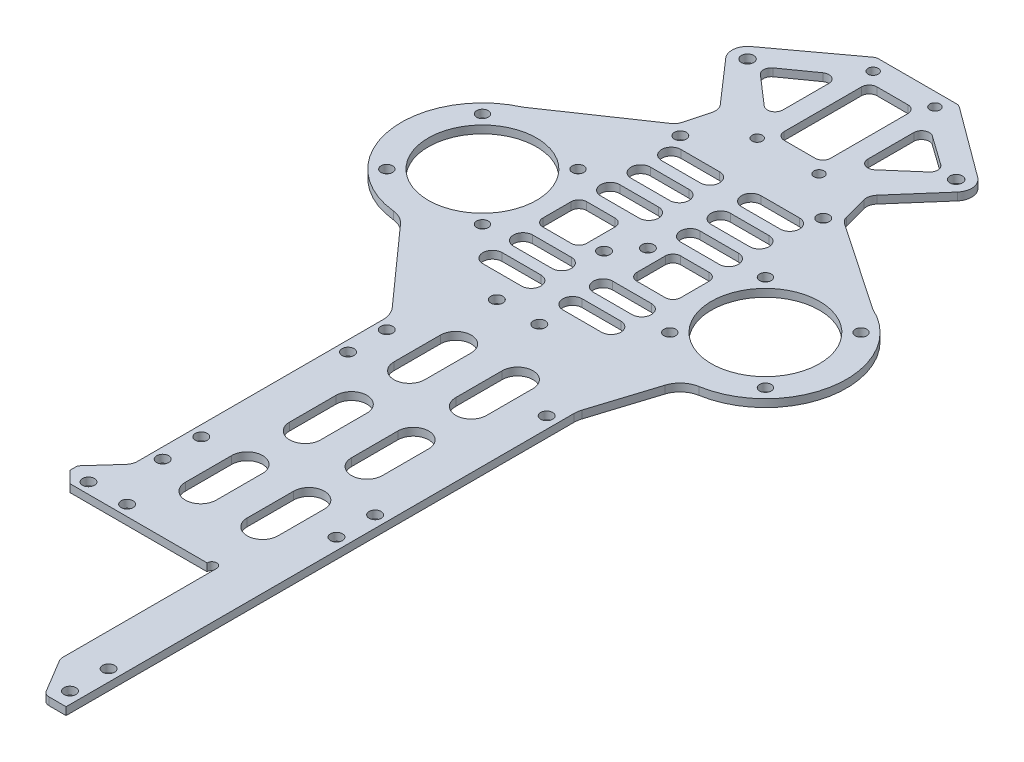
SolidWorks part; units mm, degrees
material "Thornel Mat VMA"
ref_plane "前视基准面" through (0, 0, 0) normal (0, 0, 1) x (1, 0, 0)
ref_plane "上视基准面" through (0, 0, 0) normal (0, 1, 0) x (1, 0, 0)
ref_plane "右视基准面" through (0, 0, 0) normal (1, 0, 0) x (0, 0, -1)
other "Configuration Table"
sketch "草图1" plane through (0, 0, 0) normal (0, 1, 0) x (1, 0, 0)
  line L0 (0, 0) -> (0.7762, 0) construction
  line L1 (0, 0) -> (0, 1.2776) construction
  line L2 (-36.625, 0) -> (-24.2506, 12.3744) construction
  line L3 (-8, 72.5) -> (-18.5, 33.1) construction
  line L4 (-18.5, 33.1) -> (-48.9994, 12.3744) construction
  line L5 (-8, 72.5) -> (8, 72.5) construction
  line L6 (-10.6894, 76) -> (10.6894, 76)
  line L7 (-10.6894, 76) -> (-21.5461, 35.2617)
  line L8 (-21.5461, 35.2617) -> (-45.2799, 19.1336)
  line L9 (-21.5461, 35.2617) -> (-50.9665, 15.2692) construction
  line L10 (-36.625, -21) -> (-15.75, -44.4)
  line L11 (21.5461, 35.2617) -> (45.2799, 19.1336)
  line L12 (10.6894, 76) -> (21.5461, 35.2617)
  line L13 (36.625, -21) -> (30, -42)
  line L15 (-15.75, -44.4) -> (-15.75, -111.4)
  line L16 (27, -42) -> (27, -52) construction
  line L17 (30, -42) -> (24, -42) construction
  line L18 (30, -42) -> (30, -52) construction
  line L19 (30, -52) -> (24, -52) construction
  line L20 (24, -42) -> (24, -52) construction
  line L21 (24, -47) -> (30, -47) construction
  line L22 (-10.6894, 76) -> (8, 76) construction
  line L23 (-13, -45.4) -> (-13, -66.4) construction
  line L24 (-16, -45.4) -> (-10, -45.4) construction
  line L25 (-16, -45.4) -> (-16, -66.4) construction
  line L26 (-16, -66.4) -> (-10, -66.4) construction
  line L27 (-10, -45.4) -> (-10, -66.4) construction
  line L29 (-15.75, -111.4) -> (-22.5, -118.9)
  line L30 (-22.5, -118.9) -> (-22.5, -123.9)
  line L31 (-22.5, -123.9) -> (18.5, -123.9)
  line L32 (18.5, -123.9) -> (18.5, -164.4)
  line L34 (24.5, -174.4) -> (30, -174.4)
  line L35 (30, -42) -> (30, -105.4)
  line L37 (30, -105.4) -> (30, -174.4)
  line L38 (18.5, -164.4) -> (24.5, -174.4)
  circle A0 centre (-36.625, 0) radius 14
  circle A2 centre (-24.2506, 12.3744) radius 1.5
  circle A3 centre (-24.2506, -12.3744) radius 1.5
  circle A4 centre (-48.9994, -12.3744) radius 1.5
  circle A5 centre (-48.9994, 12.3744) radius 1.5
  circle A6 centre (-8, 42.5) radius 1.325
  circle A7 centre (-8, 72.5) radius 1.325
  circle A8 centre (8, 42.5) radius 1.325
  circle A9 centre (8, 72.5) radius 1.325
  circle A10 centre (-18.5, 33.1) radius 1.55
  circle A11 centre (18.5, 33.1) radius 1.55
  arc A12 (-45.2799, 19.1336) -> (-36.625, -21) centre (-36.625, 0) ccw
  circle A13 centre (24.2506, -12.3744) radius 1.5
  circle A14 centre (24.2506, 12.3744) radius 1.5
  circle A15 centre (48.9994, 12.3744) radius 1.5
  circle A16 centre (48.9994, -12.3744) radius 1.5
  circle A17 centre (36.625, 0) radius 14
  arc A18 (45.2799, 19.1336) -> (36.625, -21) centre (36.625, 0) cw
  circle A19 centre (-5.5, -27.4) radius 1.55
  circle A20 centre (5.5, -27.4) radius 1.55
  circle A21 centre (27, -47) radius 1.55
  circle A22 centre (-13, -48.4) radius 1.55
  circle A23 centre (-13, -58.4) radius 1.55
  circle A24 centre (-13, -96.4) radius 1.55
  circle A25 centre (-13, -106.4) radius 1.55
  circle A26 centre (27, -91.4) radius 1.55
  circle A27 centre (27, -101.4) radius 1.55
  circle A28 centre (-7.5, -121.1) radius 1.55
  circle A29 centre (-17.5, -121.1) radius 1.55
  circle A30 centre (27, -170.4) radius 1.55
  circle A31 centre (27, -160.4) radius 1.55
  circle A32 centre (2.5, 3.7) radius 1.55
  circle A33 centre (-2.5, -2.65) radius 1.55
  point P19 (-36.625, 0)
  dimension "D1" = 36.625
  dimension "D2" = 28
  dimension "D5" = 3
  dimension "D7" = 2.65
  dimension "D8" = 8
  dimension "D10" = 30
  dimension "D11" = 3.1
  dimension "D12" = 9.4
  dimension "D13" = 18.5
  dimension "D15" = 42
  dimension "D17" = 3.1
  dimension "D18" = 27.4
  dimension "D19" = 5.5
  dimension "D25" = 3.1
  dimension "D30" = 3.1
  dimension "D31" = 3
  dimension "D32" = 10
  dimension "D33" = 38
  dimension "D34" = 10
  dimension "D35" = 10
  dimension "D36" = 5
  dimension "D16" = 42
  dimension "D37" = 6.75
  dimension "D39" = 5.5
  dimension "D40" = 2.8
  dimension "D41" = 14.7
  dimension "D43" = 10
  dimension "D45" = 4
  dimension "D50" = 10
  dimension "D51" = 29.4
  dimension "D44" = 4
  dimension "D52" = 16
  dimension "D53" = 16
  dimension "D54" = 35.75
  dimension "D3" = 45
  dimension "D4" = 17.5
  dimension "D9" = 42.5
  dimension "D20" = 30
  dimension "D21" = 45.75
  dimension "D22" = 23.4
  dimension "D23" = 6
  dimension "D24" = 10
  dimension "D26" = 21
  dimension "D27" = 6
  dimension "D28" = 0.5
  dimension "D29" = 3.4
  dimension "D38" = 5
  dimension "D42" = 12.5
  dimension "D46" = 50.5
  dimension "D47" = 11.5
  dimension "D48" = 5.5
  dimension "D49" = 10
  dimension "D14" = 3.5
  dimension "D6" = 4
extrude "凸台-拉伸1" add sketch "草图1" along normal blind 2
sketch "草图2" plane through (0, 2, 0) normal (0, 1, 0) x (1, 0, 0)
  line L0 (10.6894, 76) -> (19.2173, 44)
  line L1 (0, 0) -> (0, 115.567) construction
  line L2 (21.5461, 35.2617) -> (10.6894, 76) construction
  line L3 (19.2173, 44) -> (30.0136, 56.3697)
  line L4 (10.6894, 76) -> (29.3743, 62.2191)
  line L5 (10.6894, 76) -> (-10.6894, 76) construction
  line L6 (-19.2173, 44) -> (-30.0136, 56.3697)
  line L7 (-10.6894, 76) -> (-19.2173, 44)
  line L8 (-10.6894, 76) -> (-29.3743, 62.2191)
  circle A0 centre (27, 59) radius 1.6
  arc A1 (30.0136, 56.3697) -> (29.3743, 62.2191) centre (27, 59) ccw
  circle A2 centre (-27, 59) radius 1.6
  arc A3 (-30.0136, 56.3697) -> (-29.3743, 62.2191) centre (-27, 59) cw
  dimension "D1" = 3.2
  dimension "D2" = 27
  dimension "D3" = 17
  dimension "D4" = 8
  dimension "D5" = 32
extrude "凸台-拉伸2" add sketch "草图2" against normal blind 2
sketch "草图3" plane through (0, 2, 0) normal (0, 1, 0) x (1, 0, 0)
  line L0 (-22.5, -123.9) -> (18.5, -123.9) construction
  line L1 (18.5, -123.9) -> (18.5, -164.4) construction
  line L2 (0, 0) -> (0, 90.4554) construction
  line L3 (8, 42.5) -> (27, 59) construction
  line L4 (-6, 69.5) -> (6, 69.5)
  line L5 (-6, 69.5) -> (-6, 45.5)
  line L6 (-6, 45.5) -> (6, 45.5)
  line L7 (6, 69.5) -> (6, 45.5)
  line L8 (-6, 69.5) -> (6, 45.5) construction
  line L9 (-6, 45.5) -> (6, 69.5) construction
  line L10 (27, 59) -> (8, 72.5) construction
  line L11 (8, 72.5) -> (8, 42.5) construction
  line L12 (11, 67.915) -> (11, 47.7542)
  line L13 (11, 47.7542) -> (23.7685, 58.8426)
  line L14 (23.7685, 58.8426) -> (11, 67.915)
  line L15 (-11, 47.7542) -> (-23.7685, 58.8426)
  line L16 (-23.7685, 58.8426) -> (-11, 67.915)
  line L17 (-11, 67.915) -> (-11, 47.7542)
  line L18 (-15.35, 19.7) -> (-5.35, 19.7) construction
  line L19 (-15.35, 22.2) -> (-5.35, 22.2)
  line L20 (-15.35, 17.2) -> (-5.35, 17.2)
  line L21 (-15.35, 11.8) -> (-5.35, 11.8) construction
  line L22 (-15.35, 14.3) -> (-5.35, 14.3)
  line L23 (-15.35, 9.3) -> (-5.35, 9.3)
  line L24 (-15.35, 27.6) -> (-5.35, 27.6) construction
  line L25 (-15.35, 30.1) -> (-5.35, 30.1)
  line L26 (-15.35, 25.1) -> (-5.35, 25.1)
  line L27 (-15.35, -10.75) -> (-5.35, -10.75) construction
  line L28 (-17.85, 6.2) -> (-6.5, 6.2)
  line L29 (-17.85, 6.2) -> (-17.85, -5.15)
  line L30 (-17.85, -5.15) -> (-6.5, -5.15)
  line L31 (-6.5, 6.2) -> (-6.5, -5.15)
  line L32 (-15.35, -8.25) -> (-5.35, -8.25)
  line L33 (-15.35, -13.25) -> (-5.35, -13.25)
  line L34 (-15.35, -18.65) -> (-5.35, -18.65) construction
  line L35 (-15.35, -16.15) -> (-5.35, -16.15)
  line L36 (-15.35, -21.15) -> (-5.35, -21.15)
  line L37 (15.35, 27.6) -> (5.35, 27.6) construction
  line L38 (15.35, 30.1) -> (5.35, 30.1)
  line L39 (15.35, 25.1) -> (5.35, 25.1)
  line L40 (15.35, 19.7) -> (5.35, 19.7) construction
  line L41 (15.35, 22.2) -> (5.35, 22.2)
  line L42 (15.35, 17.2) -> (5.35, 17.2)
  line L43 (15.35, 11.8) -> (5.35, 11.8) construction
  line L44 (15.35, 14.3) -> (5.35, 14.3)
  line L45 (15.35, 9.3) -> (5.35, 9.3)
  line L46 (17.85, 6.2) -> (6.5, 6.2)
  line L47 (6.5, 6.2) -> (6.5, -5.15)
  line L48 (17.85, -5.15) -> (6.5, -5.15)
  line L49 (17.85, 6.2) -> (17.85, -5.15)
  line L50 (15.35, -10.75) -> (5.35, -10.75) construction
  line L51 (15.35, -8.25) -> (5.35, -8.25)
  line L52 (15.35, -13.25) -> (5.35, -13.25)
  line L53 (15.35, -18.65) -> (5.35, -18.65) construction
  line L54 (15.35, -16.15) -> (5.35, -16.15)
  line L55 (15.35, -21.15) -> (5.35, -21.15)
  line L56 (7.125, -164.9002) -> (7.125, -36.8516) construction
  line L57 (-15.75, -44.4) -> (-15.75, -111.4) construction
  line L58 (-0.875, -42.65) -> (-0.875, -54.65) construction
  line L61 (3.125, -42.65) -> (3.125, -54.65)
  line L64 (-4.875, -42.65) -> (-4.875, -54.65)
  line L67 (-0.875, -69.65) -> (-0.875, -81.65) construction
  line L68 (3.125, -69.65) -> (3.125, -81.65)
  line L69 (-4.875, -69.65) -> (-4.875, -81.65)
  line L70 (-0.875, -96.65) -> (-0.875, -108.65) construction
  line L71 (3.125, -96.65) -> (3.125, -108.65)
  line L72 (-4.875, -96.65) -> (-4.875, -108.65)
  line L73 (15.125, -96.65) -> (15.125, -108.65) construction
  line L74 (11.125, -96.65) -> (11.125, -108.65)
  line L75 (19.125, -96.65) -> (19.125, -108.65)
  line L76 (15.125, -69.65) -> (15.125, -81.65) construction
  line L77 (11.125, -69.65) -> (11.125, -81.65)
  line L78 (19.125, -69.65) -> (19.125, -81.65)
  line L79 (15.125, -42.65) -> (15.125, -54.65) construction
  line L80 (11.125, -42.65) -> (11.125, -54.65)
  line L81 (19.125, -42.65) -> (19.125, -54.65)
  circle A0 centre (17.25, -123.9) radius 1.25
  circle A1 centre (8, 72.5) radius 1.325 construction
  circle A2 centre (8, 42.5) radius 1.325 construction
  arc A3 (-15.35, 22.2) -> (-15.35, 17.2) centre (-15.35, 19.7) ccw
  arc A4 (-5.35, 17.2) -> (-5.35, 22.2) centre (-5.35, 19.7) ccw
  arc A5 (-15.35, 14.3) -> (-15.35, 9.3) centre (-15.35, 11.8) ccw
  arc A6 (-5.35, 9.3) -> (-5.35, 14.3) centre (-5.35, 11.8) ccw
  arc A7 (-15.35, 30.1) -> (-15.35, 25.1) centre (-15.35, 27.6) ccw
  arc A8 (-5.35, 25.1) -> (-5.35, 30.1) centre (-5.35, 27.6) ccw
  arc A9 (-15.35, -8.25) -> (-15.35, -13.25) centre (-15.35, -10.75) ccw
  arc A10 (-5.35, -13.25) -> (-5.35, -8.25) centre (-5.35, -10.75) ccw
  circle A11 centre (-2.5, -2.65) radius 1.55 construction
  circle A12 centre (2.5, 3.7) radius 1.55 construction
  circle A13 centre (-18.5, 33.1) radius 1.55 construction
  arc A14 (-15.35, -16.15) -> (-15.35, -21.15) centre (-15.35, -18.65) ccw
  arc A15 (-5.35, -21.15) -> (-5.35, -16.15) centre (-5.35, -18.65) ccw
  arc A16 (15.35, 30.1) -> (15.35, 25.1) centre (15.35, 27.6) cw
  arc A17 (5.35, 25.1) -> (5.35, 30.1) centre (5.35, 27.6) cw
  arc A18 (15.35, 22.2) -> (15.35, 17.2) centre (15.35, 19.7) cw
  arc A19 (5.35, 17.2) -> (5.35, 22.2) centre (5.35, 19.7) cw
  arc A20 (15.35, 14.3) -> (15.35, 9.3) centre (15.35, 11.8) cw
  arc A21 (5.35, 9.3) -> (5.35, 14.3) centre (5.35, 11.8) cw
  arc A22 (15.35, -8.25) -> (15.35, -13.25) centre (15.35, -10.75) cw
  arc A23 (5.35, -13.25) -> (5.35, -8.25) centre (5.35, -10.75) cw
  arc A24 (15.35, -16.15) -> (15.35, -21.15) centre (15.35, -18.65) cw
  arc A25 (5.35, -21.15) -> (5.35, -16.15) centre (5.35, -18.65) cw
  arc A32 (3.125, -42.65) -> (-4.875, -42.65) centre (-0.875, -42.65) ccw
  arc A33 (-4.875, -54.65) -> (3.125, -54.65) centre (-0.875, -54.65) ccw
  arc A34 (3.125, -69.65) -> (-4.875, -69.65) centre (-0.875, -69.65) ccw
  arc A35 (-4.875, -81.65) -> (3.125, -81.65) centre (-0.875, -81.65) ccw
  arc A36 (3.125, -96.65) -> (-4.875, -96.65) centre (-0.875, -96.65) ccw
  arc A37 (-4.875, -108.65) -> (3.125, -108.65) centre (-0.875, -108.65) ccw
  arc A38 (11.125, -96.65) -> (19.125, -96.65) centre (15.125, -96.65) cw
  arc A39 (19.125, -108.65) -> (11.125, -108.65) centre (15.125, -108.65) cw
  arc A40 (11.125, -69.65) -> (19.125, -69.65) centre (15.125, -69.65) cw
  arc A41 (19.125, -81.65) -> (11.125, -81.65) centre (15.125, -81.65) cw
  arc A42 (11.125, -42.65) -> (19.125, -42.65) centre (15.125, -42.65) cw
  arc A43 (19.125, -54.65) -> (11.125, -54.65) centre (15.125, -54.65) cw
  point P9 (0, 57.5)
  point P32 (-10.35, 19.7)
  point P37 (-10.35, 11.8)
  point P44 (-10.35, 27.6)
  point P57 (-10.35, -10.75)
  point P68 (-10.35, -18.65)
  point P79 (10.35, 27.6)
  point P86 (10.35, 19.7)
  point P93 (10.35, 11.8)
  point P104 (10.35, -10.75)
  point P111 (10.35, -18.65)
  point P120 (-0.875, -48.65)
  point P125 (-0.875, -75.65)
  point P132 (-0.875, -102.65)
  point P142 (15.125, -102.65)
  point P149 (15.125, -75.65)
  point P156 (15.125, -48.65)
  dimension "D1" = 2.5
  dimension "D8" = 2.5
  dimension "D20" = 4
  dimension "D2" = 2
  dimension "D3" = 3
  dimension "D4" = 3
  dimension "D5" = 3
  dimension "D6" = 4
  dimension "D7" = 4
  dimension "D9" = 2.5
  dimension "D10" = 2.5
  dimension "D11" = 4
  dimension "D12" = 10
  dimension "D13" = 3
  dimension "D14" = 3.1
  dimension "D15" = 2.9
  dimension "D16" = 3.1
  dimension "D17" = 2.9
  dimension "D18" = 22.875
  dimension "D19" = 8
  dimension "D21" = 12
  dimension "D22" = 30
  dimension "D23" = 27
  dimension "D24" = 27
extrude "切除-拉伸1" cut sketch "草图3" against normal blind 2
fillet "圆角1" radius 2 22 edges at (-6, 1, -45.5) (6, 1, -69.5) (6, 1, -45.5) (-6, 1, -69.5) (11, 1, -47.7542) (23.7685, 1, -58.8426) (11, 1, -67.915) (10.6894, 1, -76) (-11, 1, -47.7542) (-11, 1, -67.915) (-23.7685, 1, -58.8426) (-10.6894, 1, -76) (6.5, 1, 5.15) (17.85, 1, -6.2) (17.85, 1, 5.15) (6.5, 1, -6.2) (-6.5, 1, -6.2) (-6.5, 1, 5.15) (-17.85, 1, 5.15) (-17.85, 1, -6.2) (24.5, 1, 174.4) (18.5, 1, 164.4)
fillet "圆角2" radius 3 5 edges at (-15.75, 1, 111.4) (-21.5461, 1, -35.2617) (-19.2173, 1, -44) (21.5461, 1, -35.2617) (19.2173, 1, -44)
fillet "圆角3" radius 6 4 edges at (30, 1, 42) (36.625, 1, 21) (-15.75, 1, 44.4) (-36.625, 1, 21)
chamfer "倒角1" distance 3 angle 45 1 edges at (-22.5, 1, 123.9)
